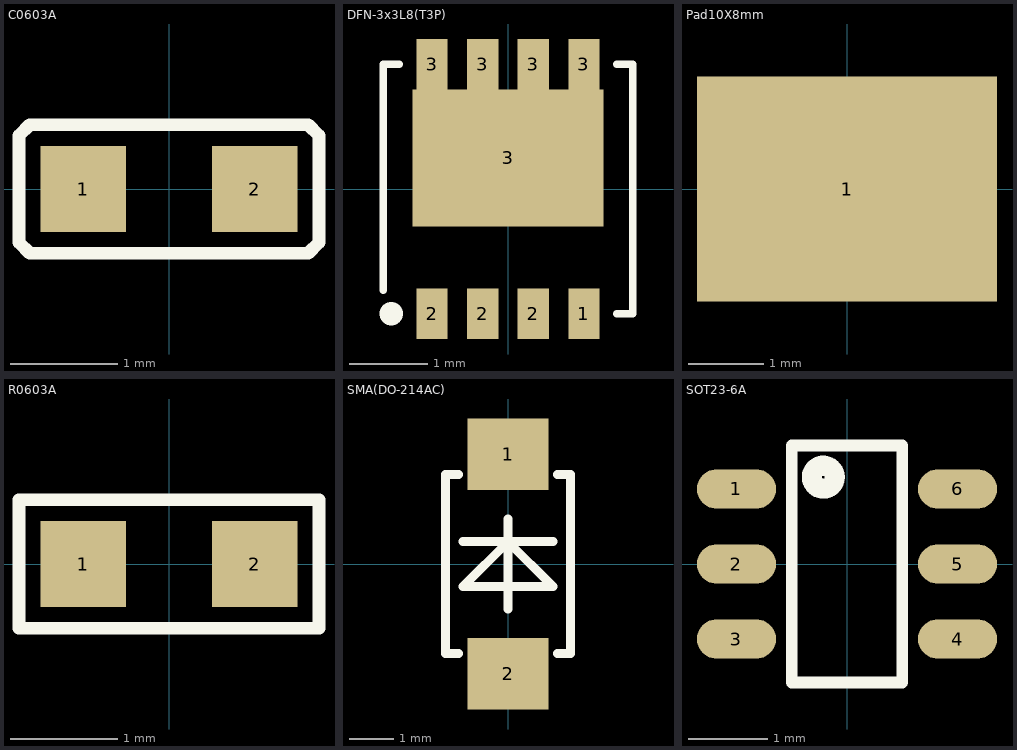
[diagram p0: the footprints below, top view; thin cyan lines are the x and y axes]
# Altium footprint library MISC82114.PcbLib: 6 footprints
Each footprint in its own frame and in the unit in brackets; x right, y up, seen from the top. Pads: shape width x height; smd on the part's side, far side on the other; paste and mask are expansions set on the pad; w line width, h text height; cw(c..) or ccw(c..) is an arc to the next point about the centre after c.

## C0603A [mm] "SMD capacitor"
pads (2):
  rect 0.8x0.8 smd mask+0.08: 1(-0.8,0) 2(0.8,0)
Top Overlay:
  lines w0.12: 0.551,-0.6 1.2,-0.6 ; -1.4,-0.5 -1.4,0.5 -1.3,0.6 1.3,0.6 1.4,0.5 1.4,-0.5 1.3,-0.6 -1.3,-0.6 -1.4,-0.5

## DFN-3x3L8(T3P) [mm] "SMD MOSFET"
height 2.5
pads (9):
  rect 0.4x0.65 smd: 1(0.975,-1.6) 2(-0.975,-1.6) 2(-0.325,-1.6) 2(0.325,-1.6) 3(-0.975,1.6) 3(-0.325,1.6) 3(0.325,1.6) 3(0.975,1.6)
  rect 2.45x1.76 smd: 3(0,0.4)
Top Overlay:
  lines w0.1: -1.6,-1.3 -1.6,1.6 -1.4,1.6 ; 1.4,-1.6 1.6,-1.6 1.6,1.6 1.4,1.6
  lines w0.3: -1.5,-1.6 -1.5,-1.597

## Pad10X8mm [mm]
pads (1):
  rect 4x3 smd: 1(0,0)

## R0603A [mm] "SMD resistor"
height 0.5
pads (2):
  rect 0.8x0.8 smd mask+0.08: 1(-0.8,0) 2(0.8,0)
Top Overlay:
  lines w0.12: -1.4,-0.6 1.4,-0.6 1.4,0.6 -1.4,0.6 -1.4,-0.6

## SMA(DO-214AC) [mm] "SMD diode"
pads (2):
  rect 1.8x1.6 smd: 1(0,2.45) 2(0,-2.45)
Top Overlay:
  lines w0.2: -1.1,-2 -1.4,-2 -1.4,2 -1.1,2 ; -1,0.5 1,0.5 ; 0,-1 0,1 ; 1.1,-2 1.4,-2 1.4,2 1.1,2 ; -1,-0.5 1,-0.5 0,0.5 -1,-0.5

## SOT23-6A [mm]
pads (6):
  oval 1x0.5 smd mask+0.05: 1(-1.4,0.95) 2(-1.4,0) 3(-1.4,-0.95) 4(1.4,-0.95) 5(1.4,0) 6(1.4,0.95)
Top Overlay:
  circle w0.254: c-0.3,1.1 r0.146
  lines w0.15: -0.7,-1.5 0.7,-1.5 0.7,1.5 -0.7,1.5 -0.7,-1.5